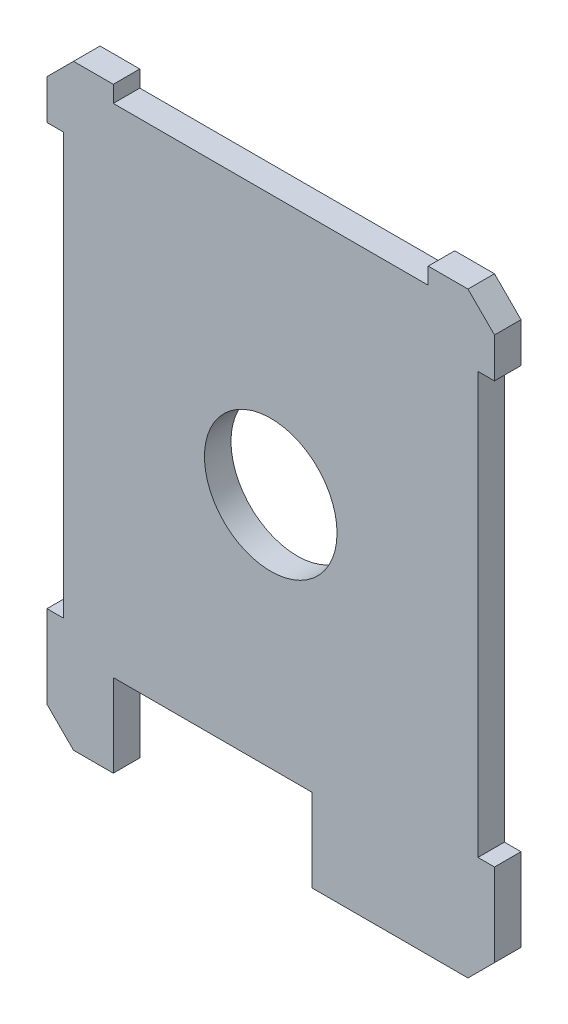
from build123d import *

# Parameters (mm, degrees)
SKETCH_1_W          = 135
SKETCH_1_H          = 180
EXTRUDE_1_DEPTH     = 8
CUT_EXTRUDE_1_REACH = 114.784
SKETCH_2_W          = 95
SKETCH_2_H          = 5
SKETCH_2_W_2        = 60
SKETCH_2_H_2        = 25
SKETCH_2_W_3        = 5
SKETCH_2_H_3        = 127
CHAMFER_1_SIZE      = 8
CUT_EXTRUDE_2_REACH = 114.784
SKETCH_3_R          = 20


with BuildPart() as part:
    # 草图1 → 凸台-拉伸1 (new body)
    with BuildSketch(Plane.XY):
        Rectangle(SKETCH_1_W, SKETCH_1_H)
    extrude(amount=EXTRUDE_1_DEPTH)

    # 草图2 → 切除-拉伸1 (cut, up to next)
    with BuildSketch(Plane.XY.offset(8), mode=Mode.PRIVATE) as cut_extrude_1_sk1:
        with Locations((0, 87.5)):
            Rectangle(SKETCH_2_W, SKETCH_2_H)
    cut_extrude_1_tool1 = extrude(cut_extrude_1_sk1.sketch, amount=-CUT_EXTRUDE_1_REACH, mode=Mode.PRIVATE) & part.part
    # 草图2 → 切除-拉伸1 (cut, up to next)
    with BuildSketch(Plane.XY.offset(8), mode=Mode.PRIVATE) as cut_extrude_1_sk2:
        with Locations((-17.5, -77.5)):
            Rectangle(SKETCH_2_W_2, SKETCH_2_H_2)
    cut_extrude_1_tool2 = extrude(cut_extrude_1_sk2.sketch, amount=-CUT_EXTRUDE_1_REACH, mode=Mode.PRIVATE) & part.part
    # 草图2 → 切除-拉伸1 (cut, up to next)
    with BuildSketch(Plane.XY.offset(8), mode=Mode.PRIVATE) as cut_extrude_1_sk3:
        with Locations((-65, 6.5)):
            Rectangle(SKETCH_2_W_3, SKETCH_2_H_3)
    cut_extrude_1_tool3 = extrude(cut_extrude_1_sk3.sketch, amount=-CUT_EXTRUDE_1_REACH, mode=Mode.PRIVATE) & part.part
    # 草图2 → 切除-拉伸1 (cut, up to next)
    with BuildSketch(Plane.XY.offset(8), mode=Mode.PRIVATE) as cut_extrude_1_sk4:
        with Locations((65, 6.5)):
            Rectangle(SKETCH_2_W_3, SKETCH_2_H_3)
    cut_extrude_1_tool4 = extrude(cut_extrude_1_sk4.sketch, amount=-CUT_EXTRUDE_1_REACH, mode=Mode.PRIVATE) & part.part
    add(cut_extrude_1_tool1.solids().sort_by_distance((0, 87.5, 8))[0], mode=Mode.SUBTRACT)
    add(cut_extrude_1_tool2.solids().sort_by_distance((-17.5, -77.5, 8))[0], mode=Mode.SUBTRACT)
    add(cut_extrude_1_tool3.solids().sort_by_distance((-65, 6.5, 8))[0], mode=Mode.SUBTRACT)
    add(cut_extrude_1_tool4.solids().sort_by_distance((65, 6.5, 8))[0], mode=Mode.SUBTRACT)

    # 倒角1
    chamfer_1_edges = [part.edges().sort_by_distance(p)[0] for p in [
        (67.5, -90, 4),
        (-67.5, -90, 4),
        (-67.5, 90, 4),
        (67.5, 90, 4),
    ]]
    chamfer(chamfer_1_edges, length=CHAMFER_1_SIZE)

    # 草图3 → 切除-拉伸2 (cut, up to next)
    with BuildSketch(Plane.XY.offset(8), mode=Mode.PRIVATE) as cut_extrude_2_sk1:
        with Locations((0, 6.5)):
            Circle(SKETCH_3_R)
    cut_extrude_2_tool1 = extrude(cut_extrude_2_sk1.sketch, amount=-CUT_EXTRUDE_2_REACH, mode=Mode.PRIVATE) & part.part
    add(cut_extrude_2_tool1.solids().sort_by_distance((0, 6.5, 8))[0], mode=Mode.SUBTRACT)


solid = part.part
